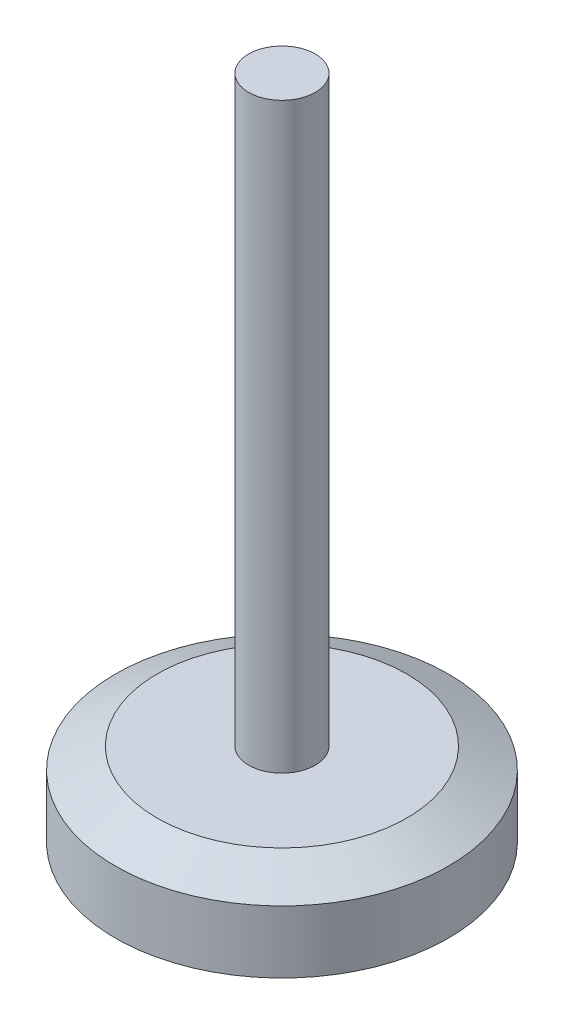
from build123d import *


with BuildPart() as part:
    # 草图1 → 旋转1 (revolve)
    with BuildSketch(Plane.XY, mode=Mode.PRIVATE) as revolve_1_sk:
        Polygon((0, 0), (40, 0), (40, 15), (30, 20), (8, 20), (8, 160), (0, 160), align=None)
    revolve(revolve_1_sk.sketch.rotate(Axis((0, 0, 0), (0, 1, 0)), 90), axis=Axis((0, 0, 0), (0, 1, 0)))


solid = part.part
